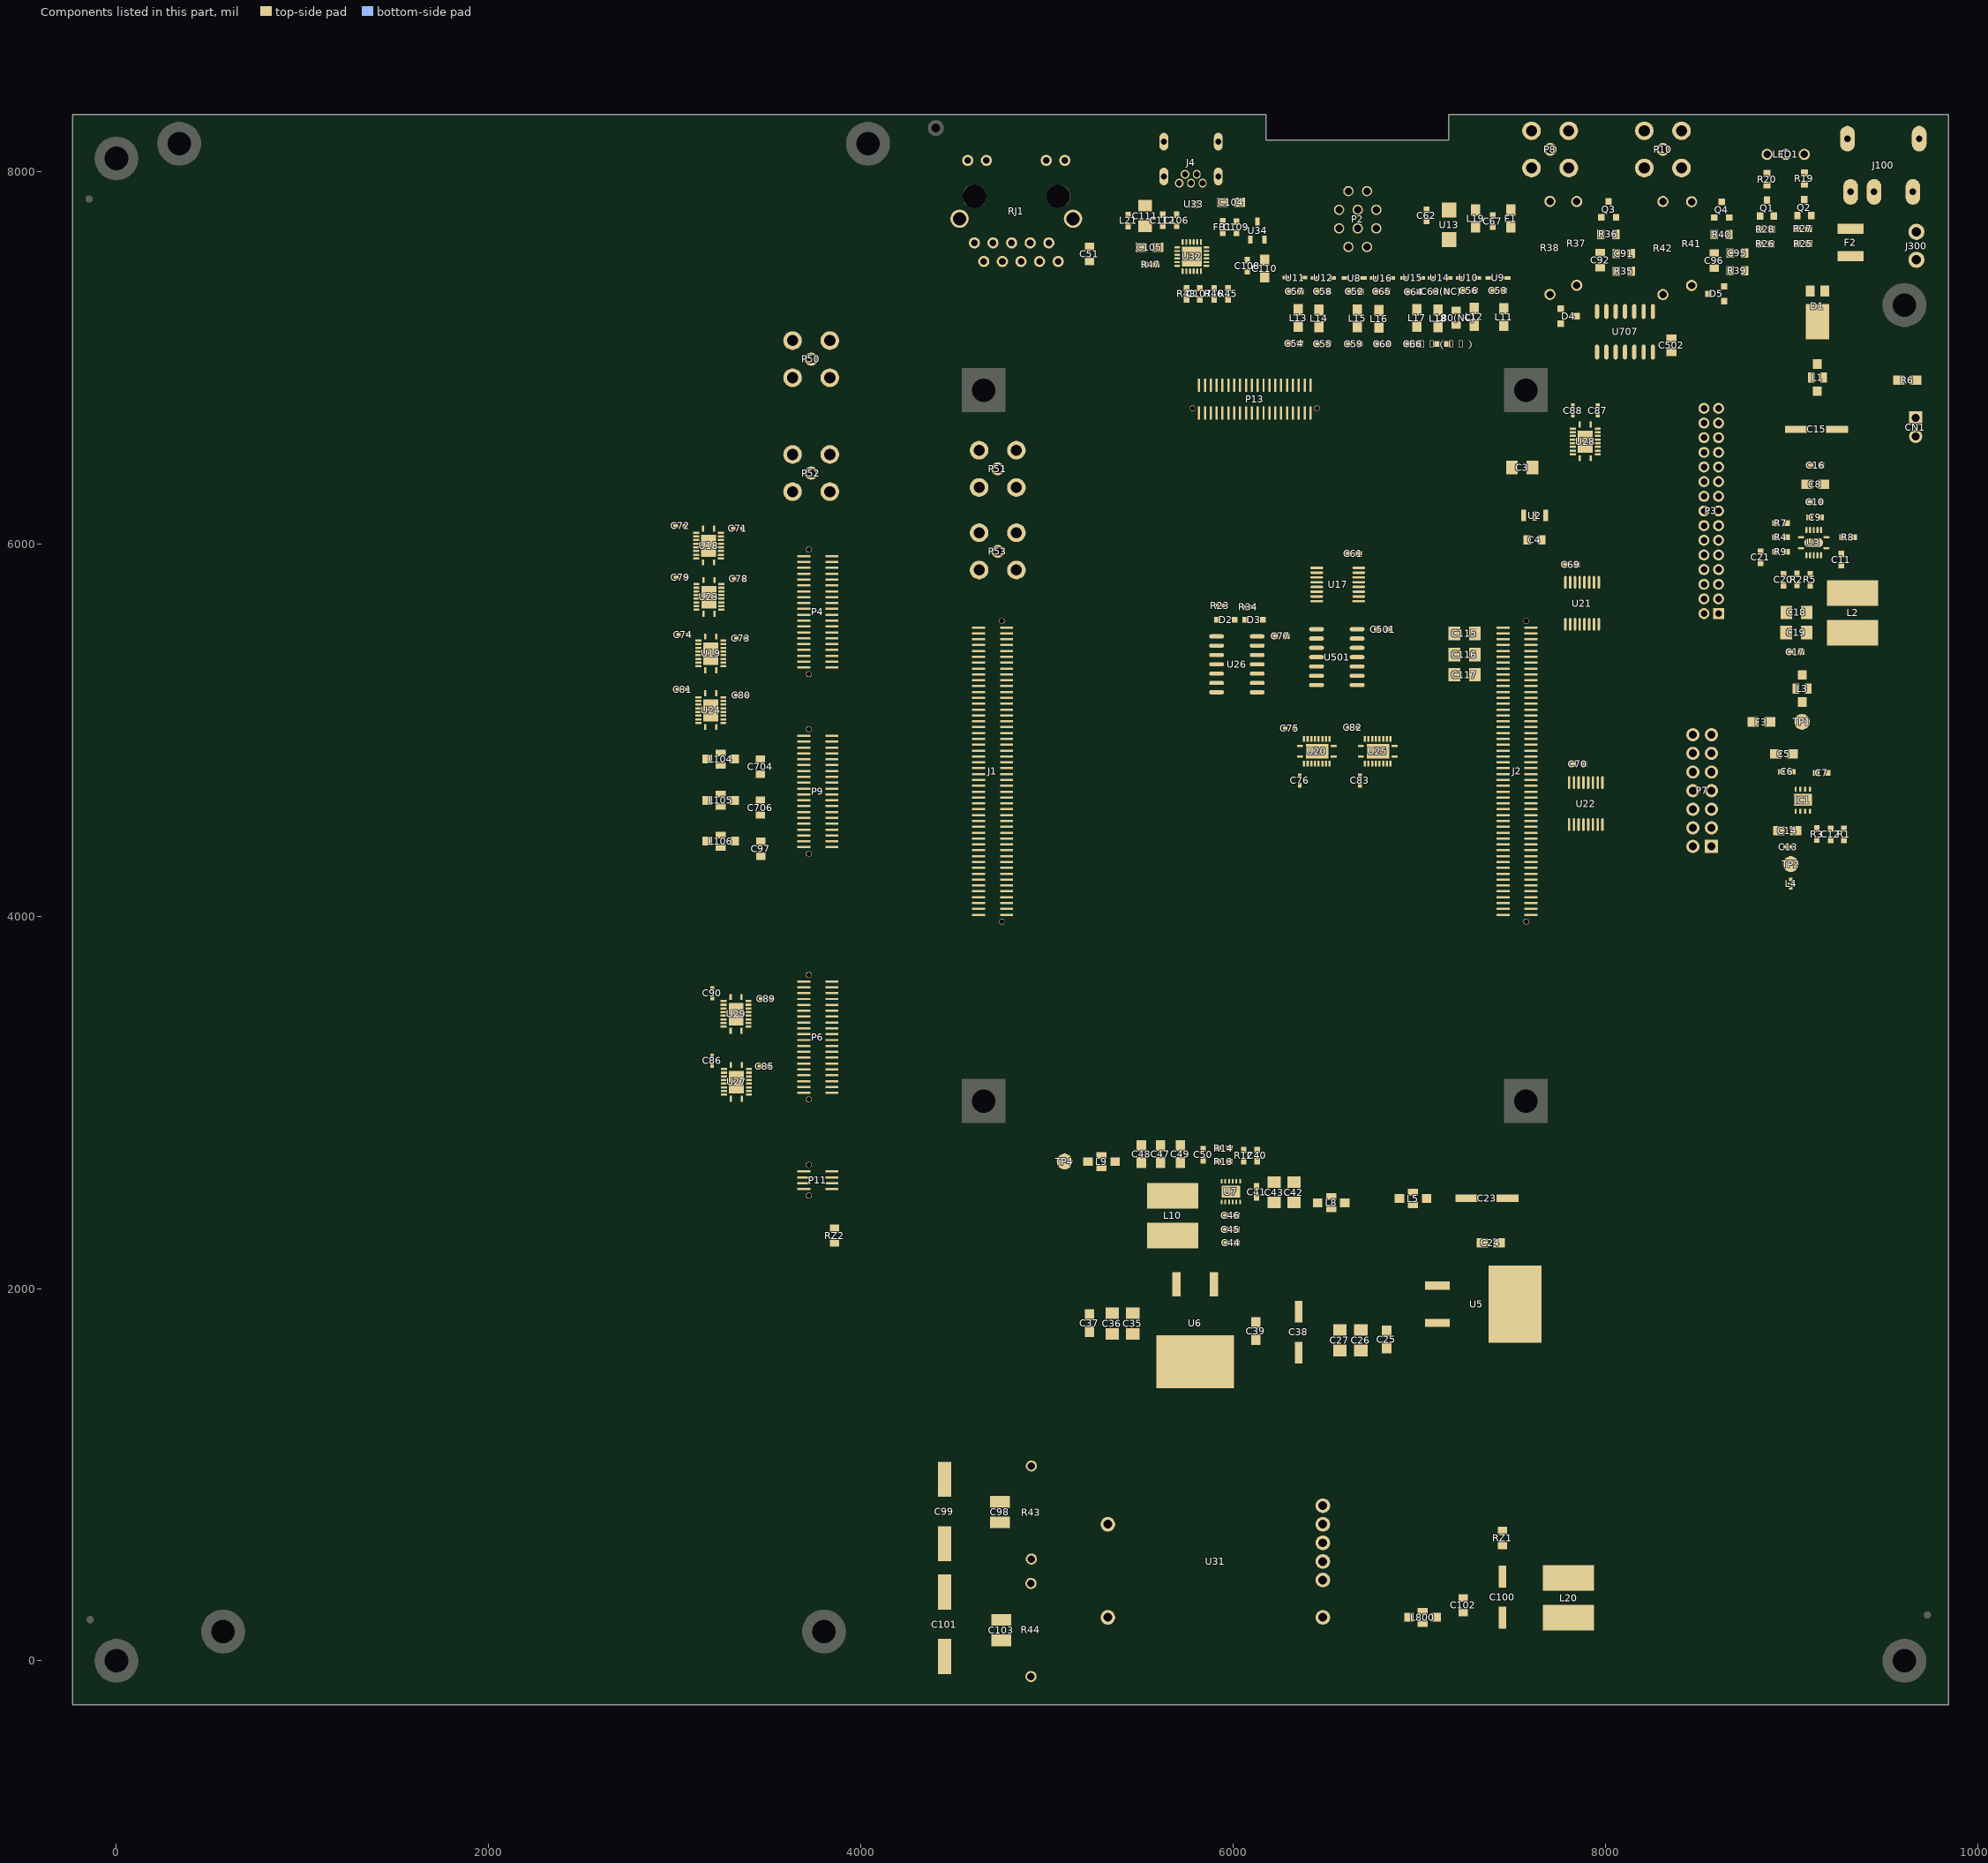
[diagram p0: the components of this part, seen from the top]
# Altium PCB MISC82191.PcbDoc (part 9 of 9)
Units mil, origin at the board's own origin, x right, y up, seen from the top; angles counter-clockwise.
Board outline 10078.74 x 8543.31 mil, 4 copper layers (Top Layer, GND, POWER, Bottom Layer); 238 components, 299 nets, 1297 pads, 1665 vias.

## Polygon pours and split planes (outlines as drawn) (continued)
NetC105_1 on Bottom Layer "Bottom Layer-No Net" (solid, remove dead copper, pour order 1107): 35 vertices, not listed, extent 5613.78,7567.16 5921.78,7753.16
HGND on Bottom Layer "Bottom Layer-No Net" (solid, remove dead copper, pour order 1006): 51 vertices, not listed, extent 3771.78,-178.59 6543.78,2203.41
DGND on Bottom Layer "Bottom Layer-No Net" (solid, remove dead copper, pour order 1007): 53 vertices, not listed, extent -1001.22,516.41 10240.78,8712.41
DGND on GND (split plane): 62 vertices, not listed, extent -216.12,508.41 9822.42,8286.99
DGND on GND (split plane): -206.69,-216.12 -216.12,-216.12 -216.12,-206.69
3V3 on POWER (split plane): 164 vertices, not listed, extent 1444.09,2543.5 9252.69,8286.99
13V on POWER (split plane): 118 vertices, not listed, extent 2907.87,508.5 9822.42,7125.32
D5V on POWER (split plane): 112 vertices, not listed, extent 3245.87,4338.5 9822.42,8286.99
DGND on POWER (split plane): 1423.91,2682.5 -216.12,2682.5 -216.12,8286.99 1423.91,8286.99
-5.4V on POWER (split plane): 24 vertices, not listed, extent 2936.87,2606.5 5156.69,4877.91

## Keep-outs
Keep-Out Layer:
  lines w5: -236.22,-236.22 -236.22,8307.09 6175.79,8307.09 6175.79,8169.29 7157.25,8169.29 7157.25,8307.09 9842.52,8307.09 9842.52,-236.22 -236.22,-236.22 ; 3109.78,-31.22 3109.78,2599.78 3357.78,2847.78 3965.78,2847.78 4102.78,2710.78 4102.78,1489.78 4297.78,1294.78 5267.78,1294.78 5596.78,965.78 5596.78,53.78 5574.78,31.78 5490.78,31.78 5470.78,51.78 5470.78,899.78 5187.78,1182.78 4244.78,1182.78 3990.78,1436.78 3990.78,2669.78 3911.78,2748.78 3442.78,2748.78 3240.78,2546.78 3240.78,-30.22 3220.78,-50.22 3128.78,-50.22 3109.78,-31.22

## Other copper
GND (plane layer: these items are gaps in the copper):
  rectangle: 4504,7444 5164,8304
  region: -217.22,-205.59 -200.22,-222.59 9832.78,-222.59 9850.78,-204.59 9850.78,506.41 9848.78,508.41 7694.78,508.41 7694.78,510.41 7551.78,653.41 7118.78,653.41 7057.78,714.41 7057.78,1054.41 7034.78,1077.41 5492.78,1077.41 5554.78,1016.41 5555.78,1007.41 5579.78,1000.41 5601.78,978.41 5601.78,73.41 5575.78,47.41 5505.78,47.41 5477.78,75.41 5477.78,908.41 5189.78,1196.41 4255.78,1196.41 3997.78,1454.41 3997.78,2688.41 3921.78,2764.41 3450.78,2764.41 3243.78,2557.41 3243.78,-13.59 3220.78,-36.59 3138.78,-36.59 3115.78,-13.59 3115.78,2608.41 3122.78,2612.41 3193.78,2682.41 -212.22,2682.41 -217.22,2677.41
POWER (plane layer: these items are gaps in the copper):
  region: -221.22,-216.59 -204.22,-233.59 9828.78,-233.59 9846.78,-215.59 9846.78,495.41 9844.78,497.41 7690.78,497.41 7690.78,499.41 7547.78,642.41 7114.78,642.41 7053.78,703.41 7057.78,1054.41 7034.78,1077.41 5512.78,1077.41 5575.78,1008.41 5575.78,989.41 5597.78,967.41 5597.78,62.41 5571.78,36.41 5501.78,36.41 5473.78,64.41 5473.78,897.41 5185.78,1185.41 4251.78,1185.41 3993.78,1443.41 3993.78,2677.41 3917.78,2753.41 3446.78,2753.41 3239.78,2546.41 3239.78,-24.59 3216.78,-47.59 3134.78,-47.59 3111.78,-24.59 3111.78,2597.41 3171.78,2683.41 3163.78,2682.41 3036.78,2682.41 -216.22,2671.41 -221.22,2666.41
  lines w20: -227.22,2672.41 3037.78,2672.41 3101.78,2608.41 3114.78,2608.41 ; 1434,2674.41 1434,8307.09 ; 2965.78,4514.41 2962.78,4514.41 2897.78,4449.41 2897.78,4203.41 3065.78,4035.41 3666.78,4035.41 3964.78,3737.41 3964.78,2858.41 4107.78,2715.41 ; 4924.78,5254.41 4924.78,5256.41 5235.78,5567.41 5235.78,5990.41 5638.78,6393.41 7697.78,6393.41 7776.78,6314.41 7776.78,6035.41 7704.78,5963.41 6023.78,5963.41 5801.78,5741.41 5801.78,5104.41 6012.78,4893.41 6909.78,4893.41 ; 4927.78,5254.41 3430.78,5254.41 3344.78,5168.41 3288.78,5168.41 3235.78,5221.41 3235.78,6902.78 4003,7670 7257.37,7670 7542.78,7955.41 8978.78,7955.41 9104.78,8081.41 9104.78,8308.41 ; 5072.78,2601.41 5073.78,2601.41 5141.78,2533.41 6354.78,2533.41 7182.78,3361.41 8990.78,3361.41 9262.78,3633.41 9262.78,5113.41 9094.78,5281.41 8581.78,5281.41 8350.78,5050.41 7733.78,5050.41 7520.78,5263.41 7520.78,5407.78 7601.41,5488.41 7842.78,5488.41 7987.78,5488.41 8347.78,5848.41 8347.78,6677.41 8802.78,7132.41 ; 5561.78,1008.41 5569.78,1008.41 5626.78,1065.41 7032.78,1065.41 7048.78,1049.41 7048.78,705.41 7111.78,642.41 7542.78,642.41 7607.78,577.41 7607.78,575.41 7684.78,498.41 9838.78,498.41 ; 6910.78,4893.41 6984.78,4819.41 6984.78,4538.41 7194.78,4328.41 7997.78,4328.41 8135.78,4466.41 9254.78,4466.41 ; 8805.78,7135.41 9845.78,7135.41 ; 2926.78,4557.41 2967.78,4516.41 4017.78,4516.41 4575.78,3958.41 4575.78,2924.41 4903.78,2596.41 5071.78,2596.41 5166.78,2691.41 5166.78,4178.41 4457.19,4888 2957.37,4888 2926.78,4857.41 2926.78,4855.41 2926.78,4557.41
Multi-Layer:
  pour cut-out: 4400.78,8347.16 4458.78,8289.16 4455.78,8286.16 4455.78,7471.16 4481.78,7445.16 5158.78,7445.16 5213.78,7500.16 5213.78,8382.16 5169.78,8426.16 4446.78,8426.16 4400.78,8380.16

## Silkscreen, mask and mechanical layers (free items; w line width, h text height)
Top Overlay:
  lines w5: 4501.71,2849.61 7730.06,2849.61 7730.06,6983.47 4501.71,6983.47 4501.71,2849.61
  lines w6: 3732.78,-808.29 3732.78,8636.71
  lines w10: 179.78,-236.22 179.78,8307.09 4195.53,8307.09 4195.53,-236.22 3092.48,-236.22 3092.48,-177.17 1499.08,-177.17 1499.08,-236.22 179.78,-236.22
  text "KGND" at 4416,8057 h45 r90